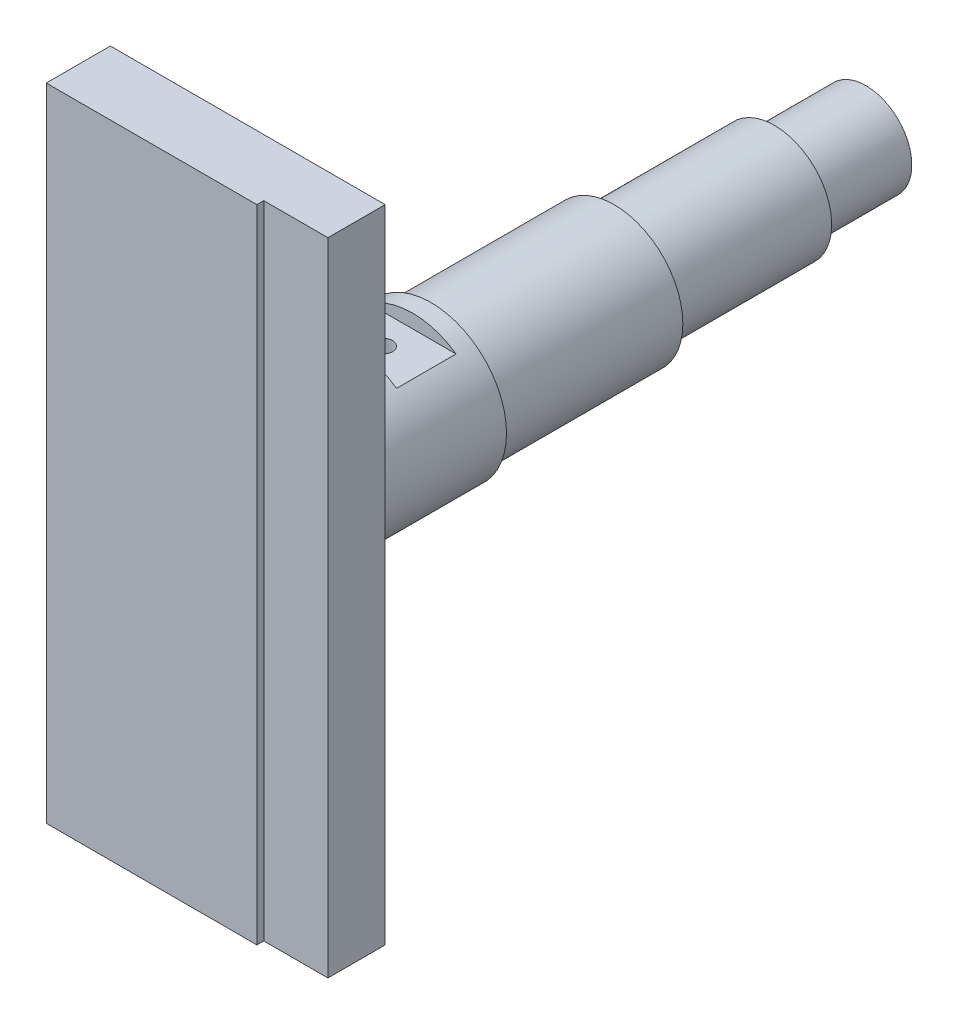
SolidWorks part; units mm, degrees
ref_plane "前视基准面" through (0, 0, 0) normal (0, 0, 1) x (1, 0, 0)
ref_plane "上视基准面" through (0, 0, 0) normal (0, 1, 0) x (1, 0, 0)
ref_plane "右视基准面" through (0, 0, 0) normal (1, 0, 0) x (0, 0, -1)
sketch "草图1" plane through (0, 0, 0) normal (0, 0, 1) x (1, 0, 0)
  circle A0 centre (0, 0) radius 15
  dimension "D1" = 30
extrude "凸台-拉伸1" add sketch "草图1" along normal blind 40
sketch "草图2" plane through (0, 0, 40) normal (0, 0, 1) x (1, 0, 0)
  circle A0 centre (0, 0) radius 16.5
  dimension "D1" = 33
extrude "凸台-拉伸2" add sketch "草图2" along normal blind 40
sketch "草图3" plane through (0, 0, 0) normal (0, 0, -1) x (-1, 0, 0)
  circle A0 centre (0, 0) radius 12.5
  dimension "D1" = 25
extrude "凸台-拉伸3" add sketch "草图3" along normal blind 35
sketch "草图4" plane through (0, 0, -35) normal (0, 0, -1) x (-1, 0, 0)
  circle A0 centre (0, 0) radius 10
  dimension "D1" = 20
extrude "凸台-拉伸4" add sketch "草图4" along normal blind 20
sketch "草图5" plane through (0, 0, 80) normal (0, 0, 1) x (1, 0, 0)
  line L1 (-30, -70) -> (30, -70)
  line L2 (-30, -70) -> (-30, 70)
  line L3 (-30, 70) -> (30, 70)
  line L4 (30, -70) -> (30, 70)
  line L5 (-30, -70) -> (30, 70) construction
  line L6 (-30, 70) -> (30, -70) construction
  point P0 (0, 0)
  dimension "D1" = 140
  dimension "D2" = 60
extrude "凸台-拉伸5" add sketch "草图5" along normal blind 14
sketch "草图6" plane through (0, 0, 94) normal (0, 0, 1) x (1, 0, 0)
  line L0 (-30, -70) -> (30, -70) construction
  line L1 (30, 70) -> (16, 70)
  line L2 (30, 70) -> (30, -70)
  line L3 (30, -70) -> (16, -70)
  line L4 (16, 70) -> (16, -70)
  dimension "D1" = 14
extrude "切除-拉伸1" cut sketch "草图6" against normal blind 1.5
sketch "草图7" plane through (0, 0, 0) normal (1, 0, 0) x (0, 0, -1)
  line L0 (-57, 16.5) -> (-57, 13.5)
  line L1 (-40, 16.5) -> (-80, 16.5) construction
  line L2 (-57, 13.5) -> (-44, 13.5)
  line L3 (-44, 13.5) -> (-44, 16.5)
  line L4 (-44, 16.5) -> (-57, 16.5)
  line L5 (-80, -16.5) -> (-80, 16.5) construction
  dimension "D1" = 23
  dimension "D2" = 13
  dimension "D3" = 3
extrude "切除-拉伸2" cut sketch "草图7" against normal mid plane 20
mirror "镜向1" about plane through (0, 0, 0) normal (0, 1, 0) of "切除-拉伸2"
hole_wizard "M5 螺纹孔1" positions "3D草图1" profile "草图8" tap size "M5" standard "GB"
sketch3d "3D草图1"
  line L0 (-9.4868, 13.5, 50.5) -> (9.4868, 13.5, 50.5)
  line L1 (-9.4868, 13.5, 57) -> (-9.4868, 13.5, 44) construction
  line L2 (9.4868, 13.5, 44) -> (9.4868, 13.5, 57) construction
  point P0 (0, 13.5, 50.5)
sketch "草图8" plane through (0, 13.5, 50.5) normal (1, 0, 0) x (0, 0, 1)
  line L0 (0, 0) -> (0, 11.2618)
  line L1 (0, 11.2618) -> (2.1, 10)
  line L2 (2.1, 10) -> (2.1, 0)
  line L5 (2.1, 0) -> (0, 0)
  line L10 (0, 11.2618) -> (-2.1, 10) construction
  line L11 (0, -6.35) -> (0, 107.95) construction
  dimension "螺纹孔钻头直径" = 4.2
  dimension "螺纹孔钻头深度" = 10
  dimension "导头角度" = 118
cosmetic thread "孔螺蚊线3" parameters "D1"=6, "D2"=5
mirror "镜向2" about plane through (0, 0, 0) normal (0, 1, 0) of "M5 螺纹孔1"
